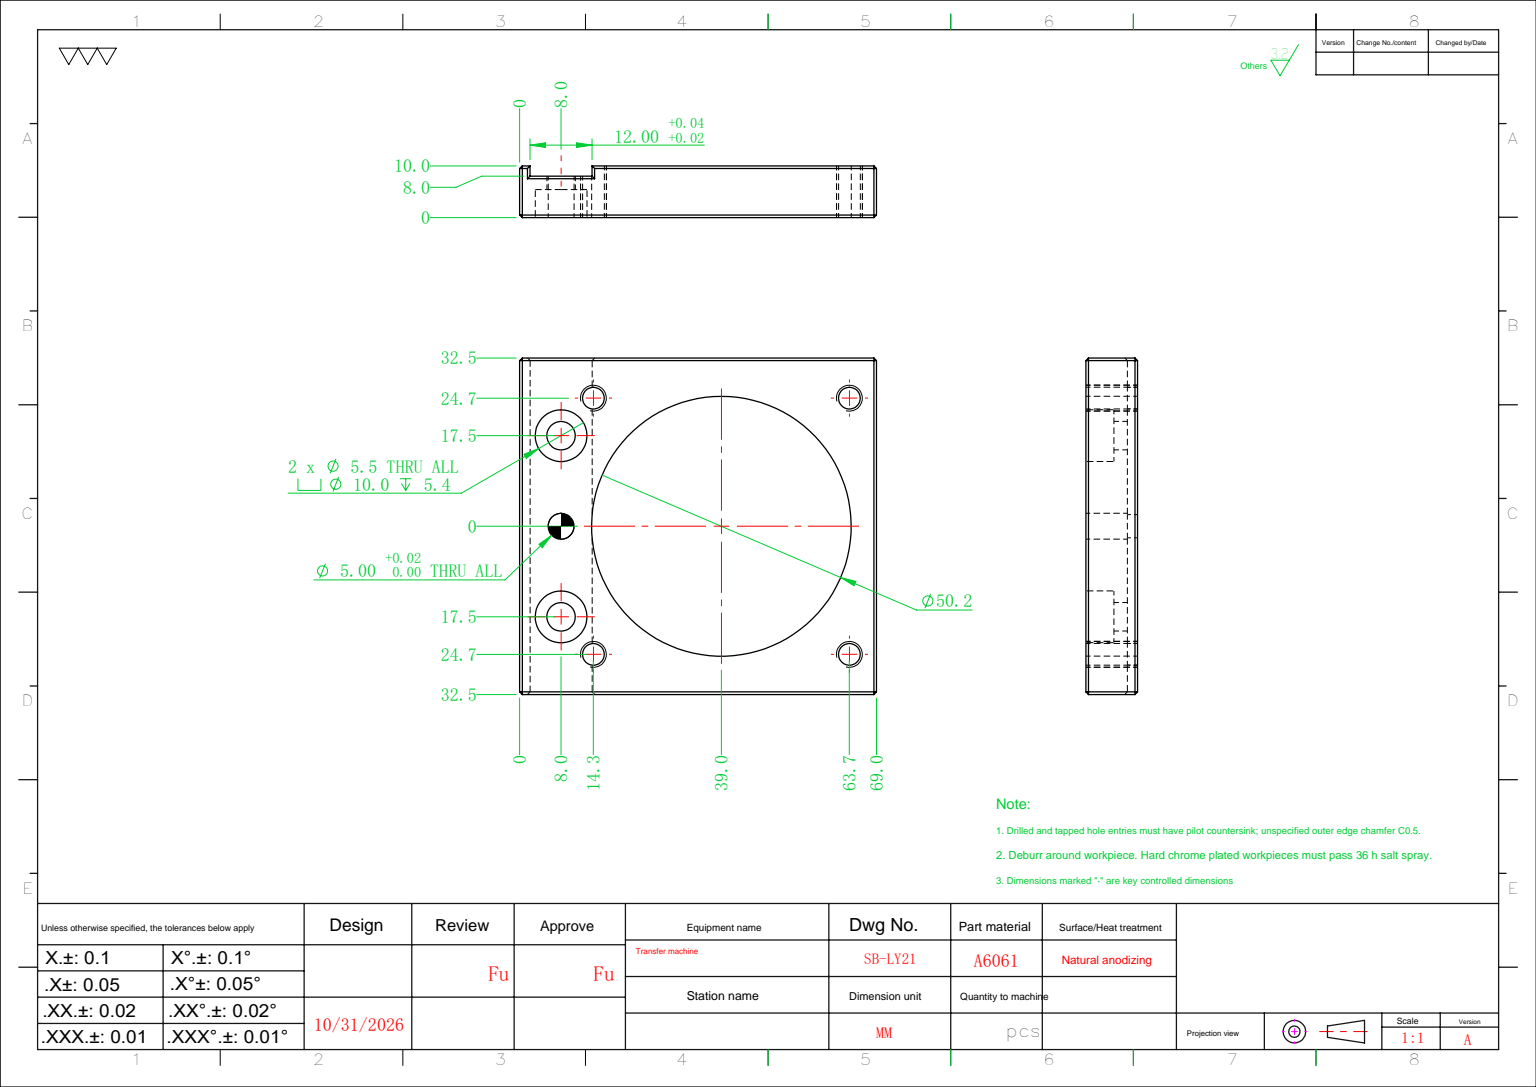
from build123d import *

# Parameters (mm, degrees)
SKETCH_1_W                     = 65
SKETCH_1_H                     = 69
EXTRUDE_1_DEPTH                = 10
SKETCH_2_W                     = 2
SKETCH_2_H                     = 12
CUT_EXTRUDE_1_DEPTH            = 75.264729179
SKETCH_3_R                     = 25.1
CUT_EXTRUDE_2_DEPTH            = 49.440685379
HOLE_WIZARD_M5_1_D             = 4.2
HOLE_WIZARD_M5_1_2_D           = 5.5
HOLE_WIZARD_M5_1_2_CBORE_D     = 10
HOLE_WIZARD_M5_1_2_CBORE_DEPTH = 5.4
MM_1_D                         = 5
CHAMFER_1_SIZE                 = 0.5


with BuildPart() as part:
    # 草图1 → 凸台-拉伸1 (new body)
    with BuildSketch(Plane.XY):
        Rectangle(SKETCH_1_W, SKETCH_1_H)
    extrude(amount=EXTRUDE_1_DEPTH)

    # 草图2 → 切除-拉伸1 (cut, through all)
    with BuildSketch(Plane.ZY.offset(32.5)):
        with Locations((1, 26.5)):
            Rectangle(SKETCH_2_W, SKETCH_2_H)
    extrude(amount=-CUT_EXTRUDE_1_DEPTH, mode=Mode.SUBTRACT)

    # 草图3 → 切除-拉伸2 (cut, through all)
    with BuildSketch(Plane.XY.offset(10)):
        with Locations((0, -4.5)):
            Circle(SKETCH_3_R)
    extrude(amount=-CUT_EXTRUDE_2_DEPTH, mode=Mode.SUBTRACT)

    # Hole Wizard M5 _1 (through all)
    with Locations(Plane.XY.offset(10)):
        with Locations((24.748737342, 20.248737342), (24.748737342, -29.248737342), (-24.748737342, -29.248737342), (-24.748737342, 20.248737342)):
            Hole(HOLE_WIZARD_M5_1_D / 2)

    # Hole Wizard M5 _1 2 (through all)
    with Locations(Plane.XY.offset(10)):
        with Locations((17.5, 26.5), (-17.5, 26.5)):
            CounterBoreHole(HOLE_WIZARD_M5_1_2_D / 2, HOLE_WIZARD_M5_1_2_CBORE_D / 2, HOLE_WIZARD_M5_1_2_CBORE_DEPTH)

    # 大小mm 暗销孔1 (through all)
    with Locations(Plane.XY.offset(10)):
        with Locations((0, 26.5)):
            Hole(MM_1_D / 2)

    # 倒角1
    chamfer_1_edges = [part.edges().sort_by_distance(p)[0] for p in [
        (-32.5, 0, 10),
        (32.5, 33.5, 0),
        (-32.5, -7, 0),
        (0, -34.5, 10),
        (32.5, 32.5, 1),
        (32.5, 26.5, 2),
        (32.5, 20.5, 1),
        (-32.5, 20.5, 1),
        (-32.5, 26.5, 2),
        (-32.5, 32.5, 1),
        (32.5, 0, 10),
        (0, -34.5, 0),
        (-32.5, 33.5, 0),
        (0, 34.5, 0),
        (32.5, -7, 0),
        (32.5, -34.5, 5),
        (-32.5, -34.5, 5),
        (-32.5, 34.5, 5),
        (32.5, 34.5, 5),
        (0, 34.5, 10),
    ]]
    chamfer(chamfer_1_edges, length=CHAMFER_1_SIZE)


solid = part.part
